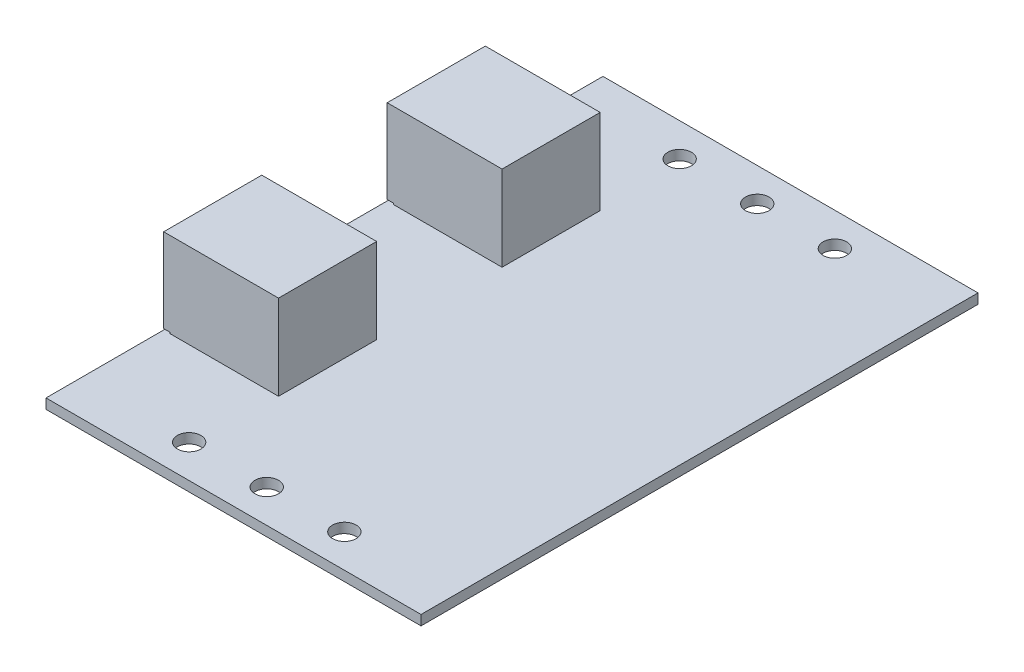
from build123d import *

# Parameters (mm, degrees)
SKETCH_1_W          = 60.4
SKETCH_1_H          = 89.7
EXTRUDE_1_DEPTH     = 1.6
SKETCH_2_R          = 1.9
CUT_EXTRUDE_1_DEPTH = 1.6
SKETCH_3_W          = 15.8
SKETCH_3_H          = 13.7
EXTRUDE_2_DEPTH     = 18.5
SKETCH_4_W          = 51.8
SKETCH_4_H          = 0.2
CUT_EXTRUDE_2_DEPTH = 1


with BuildPart() as part:
    # 草图1 → 凸台-拉伸1 (new body)
    with BuildSketch(Plane(origin=(0, 0, 0), x_dir=(1, 0, 0), z_dir=(0, 1, 0))):
        Rectangle(SKETCH_1_W, SKETCH_1_H)
    extrude(amount=EXTRUDE_1_DEPTH)

    # 草图2 → 切除-拉伸1 (cut)
    with BuildSketch(Plane(origin=(0, 1.6, 0), x_dir=(1, 0, 0), z_dir=(0, 1, 0))):
        with Locations(Location((-12.5, -39.5, 0), (0, 0, 270))):
            Circle(SKETCH_2_R)
        with Locations(Location((12.5, -39.5, 0), (0, 0, 270))):
            Circle(SKETCH_2_R)
        with Locations(Location((-12.5, 39.5, 0), (0, 0, 270))):
            Circle(SKETCH_2_R)
        with Locations(Location((12.5, 39.5, 0), (0, 0, 270))):
            Circle(SKETCH_2_R)
        with Locations(Location((0, 39.5, 0), (0, 0, 270))):
            Circle(SKETCH_2_R)
        with Locations(Location((0, -39.5, 0), (0, 0, 270))):
            Circle(SKETCH_2_R)
    extrude(amount=-CUT_EXTRUDE_1_DEPTH, mode=Mode.SUBTRACT)

    # 草图3 → 凸台-拉伸2 (add)
    with BuildSketch(Plane.ZY.offset(30.2)):
        with Locations((18, 8.45)):
            Rectangle(SKETCH_3_W, SKETCH_3_H)
        with Locations((-18, 8.45)):
            Rectangle(SKETCH_3_W, SKETCH_3_H)
    extrude(amount=-EXTRUDE_2_DEPTH)

    # 草图4 → 切除-拉伸2 (cut)
    with BuildSketch(Plane.ZY.offset(30.2)):
        with Locations((0, 1.7)):
            Rectangle(SKETCH_4_W, SKETCH_4_H)
    extrude(amount=-CUT_EXTRUDE_2_DEPTH, mode=Mode.SUBTRACT)


solid = part.part
